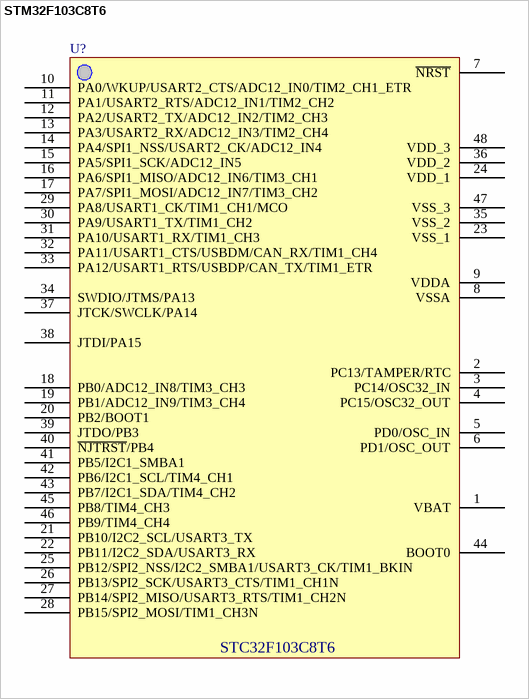
[diagram p0: symbol STM32F103C8T6]
# Altium schematic symbol library MISC82121-8.SCHLIB: 1 symbol
Pins are listed as number, name and electrical type; pins without a type are passive.


## STM32F103C8T6
designator U?
footprint LQFP48 (Footprint not found)
pins: 1 VBAT, 2 PC13/TAMPER/RTC, 3 PC14/OSC32_IN, 4 PC15/OSC32_OUT, 5 PD0/OSC_IN, 6 PD1/OSC_OUT, 7 ~{NRST}, 8 VSSA, 9 VDDA, 10 PA0/WKUP/USART2_CTS/ADC12_IN0/TIM2_CH1_ETR, 11 PA1/USART2_RTS/ADC12_IN1/TIM2_CH2, 12 PA2/USART2_TX/ADC12_IN2/TIM2_CH3, 13 PA3/USART2_RX/ADC12_IN3/TIM2_CH4, 14 PA4/SPI1_NSS/USART2_CK/ADC12_IN4, 15 PA5/SPI1_SCK/ADC12_IN5, 16 PA6/SPI1_MISO/ADC12_IN6/TIM3_CH1, 17 PA7/SPI1_MOSI/ADC12_IN7/TIM3_CH2, 18 PB0/ADC12_IN8/TIM3_CH3, 19 PB1/ADC12_IN9/TIM3_CH4, 20 PB2/BOOT1, 21 PB10/I2C2_SCL/USART3_TX, 22 PB11/I2C2_SDA/USART3_RX, 23 VSS_1, 24 VDD_1, 25 PB12/SPI2_NSS/I2C2_SMBA1/USART3_CK/TIM1_BKIN, 26 PB13/SPI2_SCK/USART3_CTS/TIM1_CH1N, 27 PB14/SPI2_MISO/USART3_RTS/TIM1_CH2N, 28 PB15/SPI2_MOSI/TIM1_CH3N, 29 PA8/USART1_CK/TIM1_CH1/MCO, 30 PA9/USART1_TX/TIM1_CH2, 31 PA10/USART1_RX/TIM1_CH3, 32 PA11/USART1_CTS/USBDM/CAN_RX/TIM1_CH4, 33 PA12/USART1_RTS/USBDP/CAN_TX/TIM1_ETR, 34 SWDIO/JTMS/PA13, 35 VSS_2, 36 VDD_2, 37 JTCK/SWCLK/PA14, 38 JTDI/PA15, 39 JTDO/PB3, 40 ~{NJTRST}/PB4, 41 PB5/I2C1_SMBA1, 42 PB6/I2C1_SCL/TIM4_CH1, 43 PB7/I2C1_SDA/TIM4_CH2, 44 BOOT0, 45 PB8/TIM4_CH3, 46 PB9/TIM4_CH4, 47 VSS_3, 48 VDD_3